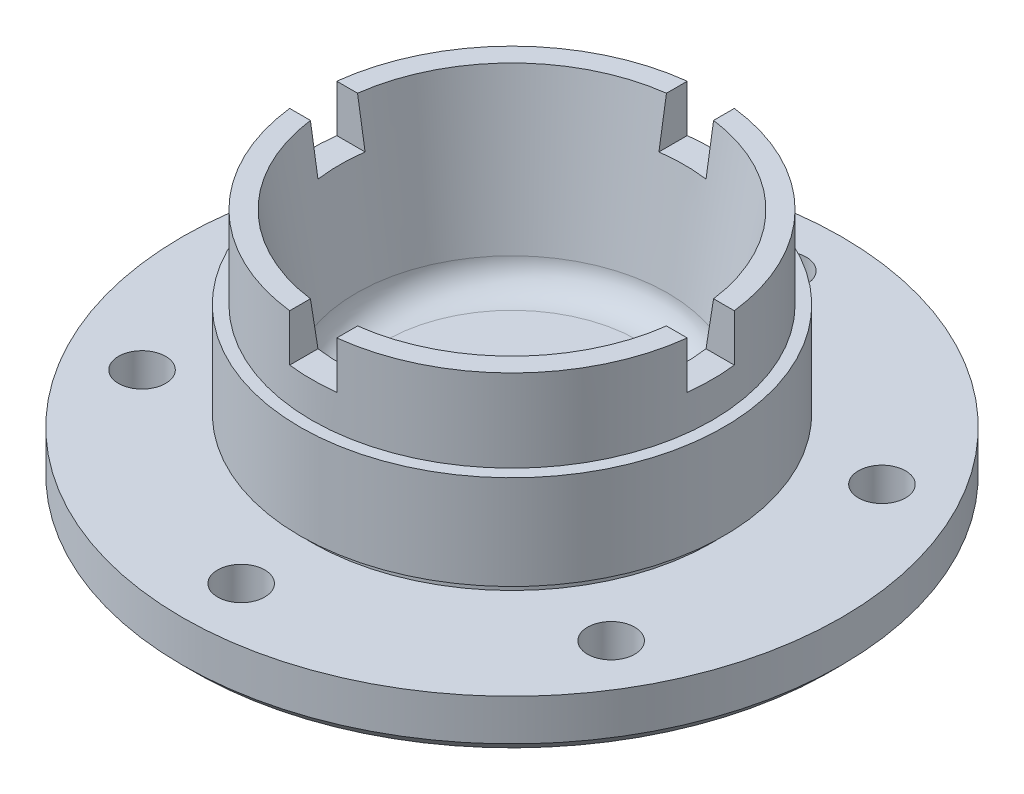
SolidWorks part; units mm, degrees
ref_plane "Front" through (0, 0, 0) normal (0, 0, 1) x (1, 0, 0)
ref_plane "Top" through (0, 0, 0) normal (0, 1, 0) x (1, 0, 0)
ref_plane "Right" through (0, 0, 0) normal (1, 0, 0) x (0, 0, -1)
sketch "Sketch1" plane through (0, 0, 0) normal (0, 0, 1) x (1, 0, 0)
  line L0 (0, 2) -> (0, 11)
  line L1 (0, 11) -> (0, 2)
  line L2 (0, 2) -> (31, 2)
  line L3 (31, 2) -> (32, 0)
  line L4 (54, 0) -> (56, 2)
  line L5 (32, 0) -> (54, 0)
  line L6 (56, 2) -> (56, 9)
  line L7 (56, 9) -> (34, 9)
  line L8 (34, 9) -> (34, 11)
  line L9 (34, 11) -> (36, 11)
  line L10 (36, 11) -> (36, 27)
  line L11 (36, 27) -> (34, 27)
  line L12 (34, 27) -> (34, 41)
  line L13 (0, 11) -> (16.5706, 11)
  line L14 (21.4751, 11) -> (16.5706, 11)
  line L15 (34, 41) -> (30.5, 41)
  line L17 (30.5, 41) -> (30.5, 56.6339)
  line L18 (30.5, 41) -> (26.4502, 15.5025)
  arc A0 (26.4502, 15.5025) -> (21.4751, 11) centre (21.4751, 16) cw
  point P8 (56, 0)
  point P21 (26, 11)
  dimension "D15" = 5
  dimension "D2" = 30.5
  dimension "D3" = 31
  dimension "D5" = 9
  dimension "D6" = 22
  dimension "D7" = 2
  dimension "D8" = 2
  dimension "D9" = 16
  dimension "D10" = 2
  dimension "D11" = 14
revolve "Revolve1" add sketch "Sketch1" angle 360 about L0
sketch "Sketch2" plane through (0, 41, 0) normal (0, 1, 0) x (1, 0, 0)
  line L0 (48.2155, 4) -> (14.6829, 4)
  line L1 (-4, 48.2155) -> (4, 48.2155)
  line L2 (-4, 48.2155) -> (-4, 14.6829)
  line L3 (-4, 14.6829) -> (4, 14.6829)
  line L4 (4, 48.2155) -> (4, 14.6829)
  line L5 (48.2155, 4) -> (48.2155, -4)
  line L6 (48.2155, -4) -> (14.6829, -4)
  line L7 (14.6829, 4) -> (14.6829, -4)
  line L8 (4, -48.2155) -> (4, -14.6829)
  line L9 (4, -48.2155) -> (-4, -48.2155)
  line L10 (-4, -48.2155) -> (-4, -14.6829)
  line L11 (4, -14.6829) -> (-4, -14.6829)
  line L12 (-48.2155, -4) -> (-14.6829, -4)
  line L13 (-48.2155, -4) -> (-48.2155, 4)
  line L14 (-48.2155, 4) -> (-14.6829, 4)
  line L15 (-14.6829, -4) -> (-14.6829, 4)
  point P20 (0, 0)
  dimension "D1" = 8
  dimension "D2" = 4
  dimension "D3" = 4
extrude "Cut-Extrude1" cut sketch "Sketch2" against normal blind 8
sketch "Sketch3" plane through (0, 41, 0) normal (0, 1, 0) x (1, 0, 0)
  line L0 (0, 0) -> (74.2039, 0) construction
  line L1 (0, 0) -> (0, 61.9256) construction
  line L2 (0, 0) -> (65.0033, 37.5297) construction
  line L3 (0, 0) -> (-58.8517, 33.978) construction
  circle A0 centre (-39.8372, -23) radius 4
  circle A1 centre (0, 46) radius 4
  circle A2 centre (39.8372, 23) radius 4
  circle A3 centre (-39.8372, 23) radius 4
  circle A4 centre (0, -46) radius 4
  circle A5 centre (39.8372, -23) radius 4
  dimension "D3" = 8
  dimension "D4" = 8
  dimension "D1" = 60
  dimension "D5" = 60
extrude "Cut-Extrude2" cut sketch "Sketch3" against normal blind 93
scale "Scale 1" bodies to scale 103 scale about centroid uniform scaling yes scale factor 1.875
